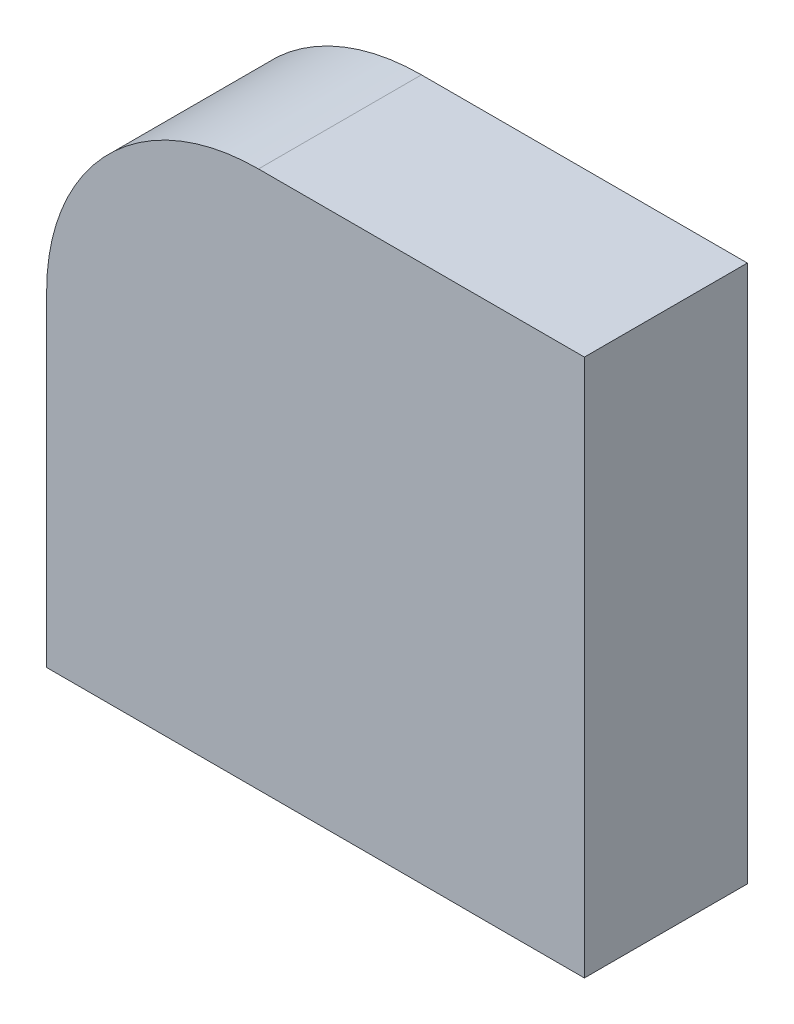
from build123d import *

# Parameters (mm, degrees)
SKETCH1_W           = 40
SKETCH1_H           = 40
BOSS_EXTRUDE1_DEPTH = 10
FILLET1_R           = 20
CUT_EXTRUDE1_DEPTH  = 58.445626465


with BuildPart() as part:
    # Sketch1 → Boss-Extrude1 (new body)
    with BuildSketch(Plane.XY):
        with Locations((20, 20)):
            Rectangle(SKETCH1_W, SKETCH1_H)
    extrude(amount=BOSS_EXTRUDE1_DEPTH)

    # Fillet1
    fillet1_edges = [part.edges().sort_by_distance(p)[0] for p in [
        (0, 40, 5),
    ]]
    fillet(fillet1_edges, radius=FILLET1_R)

    # Sketch2 → Cut-Extrude1 (cut, through all)
    with BuildSketch(Plane(origin=(0, 0, 0), x_dir=(-1, 0, 0), z_dir=(0, 0, -1))):
        with BuildLine():
            Line((-40, 40), (-20, 40))
            ThreePointArc((-20, 40), (-5.857864376, 34.142135624), (0, 20))
            Line((0, 20), (0, 0))
            Line((0, 0), (-7, 0))
            Line((-7, 0), (-7, 20))
            ThreePointArc((-7, 20), (-10.807611845, 29.192388155), (-20, 33))
            Line((-20, 33), (-40, 33))
            Line((-40, 33), (-40, 40))
        make_face()
    extrude(amount=-CUT_EXTRUDE1_DEPTH, mode=Mode.SUBTRACT)


solid = part.part
